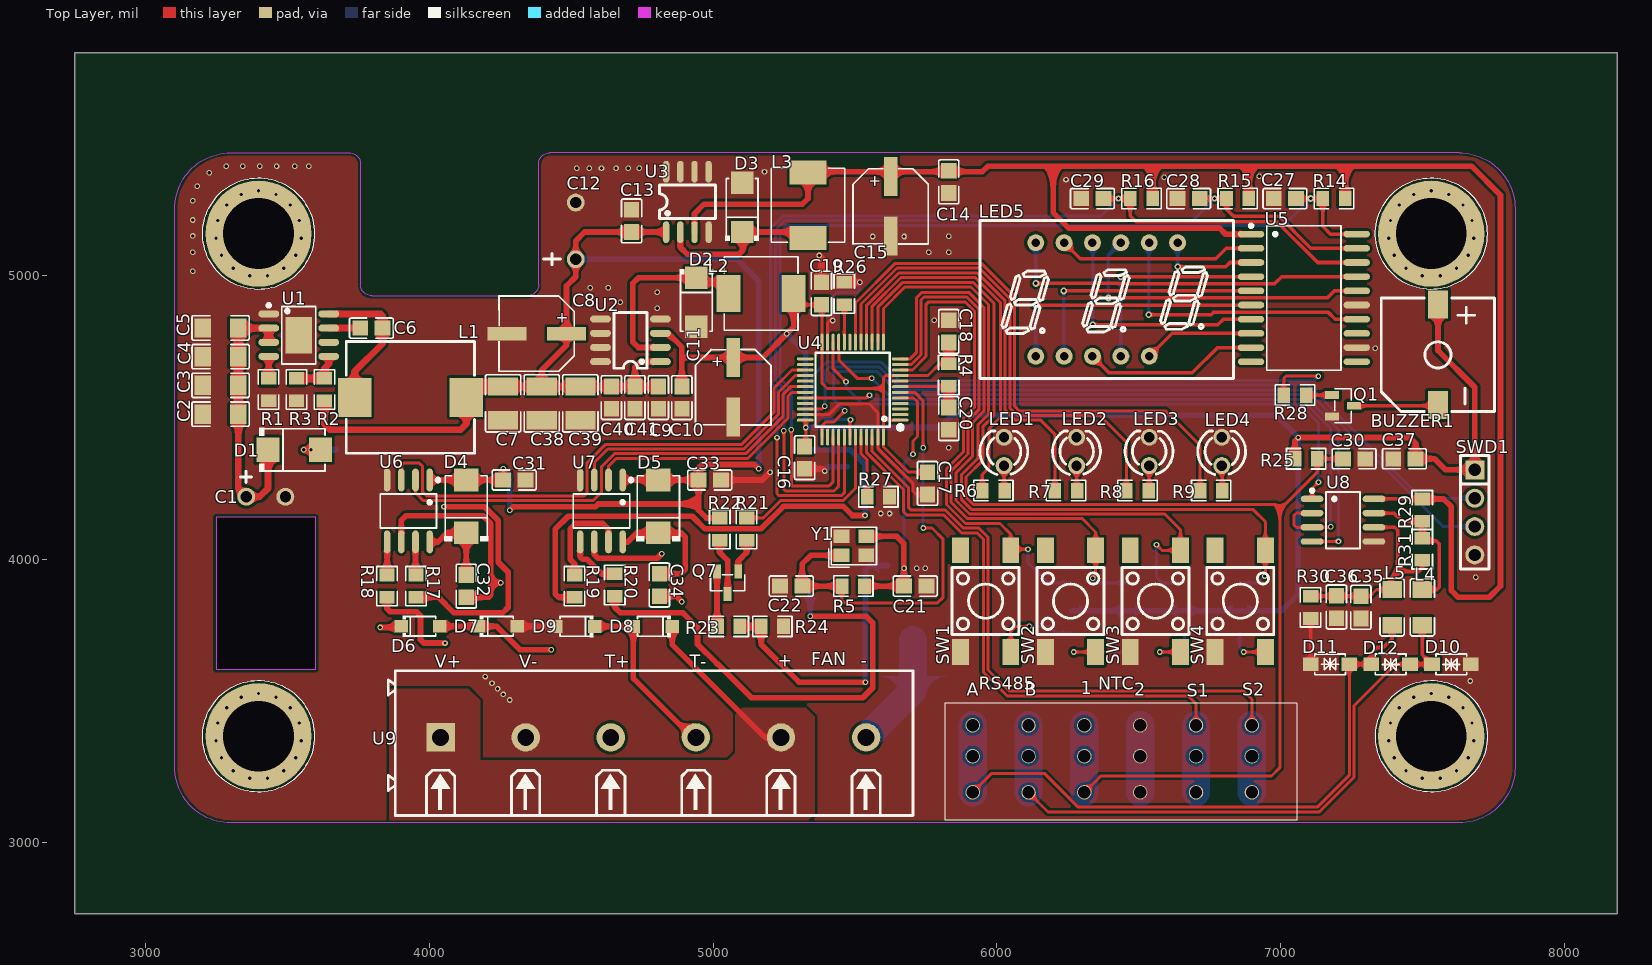
[diagram p0: Top Layer view]
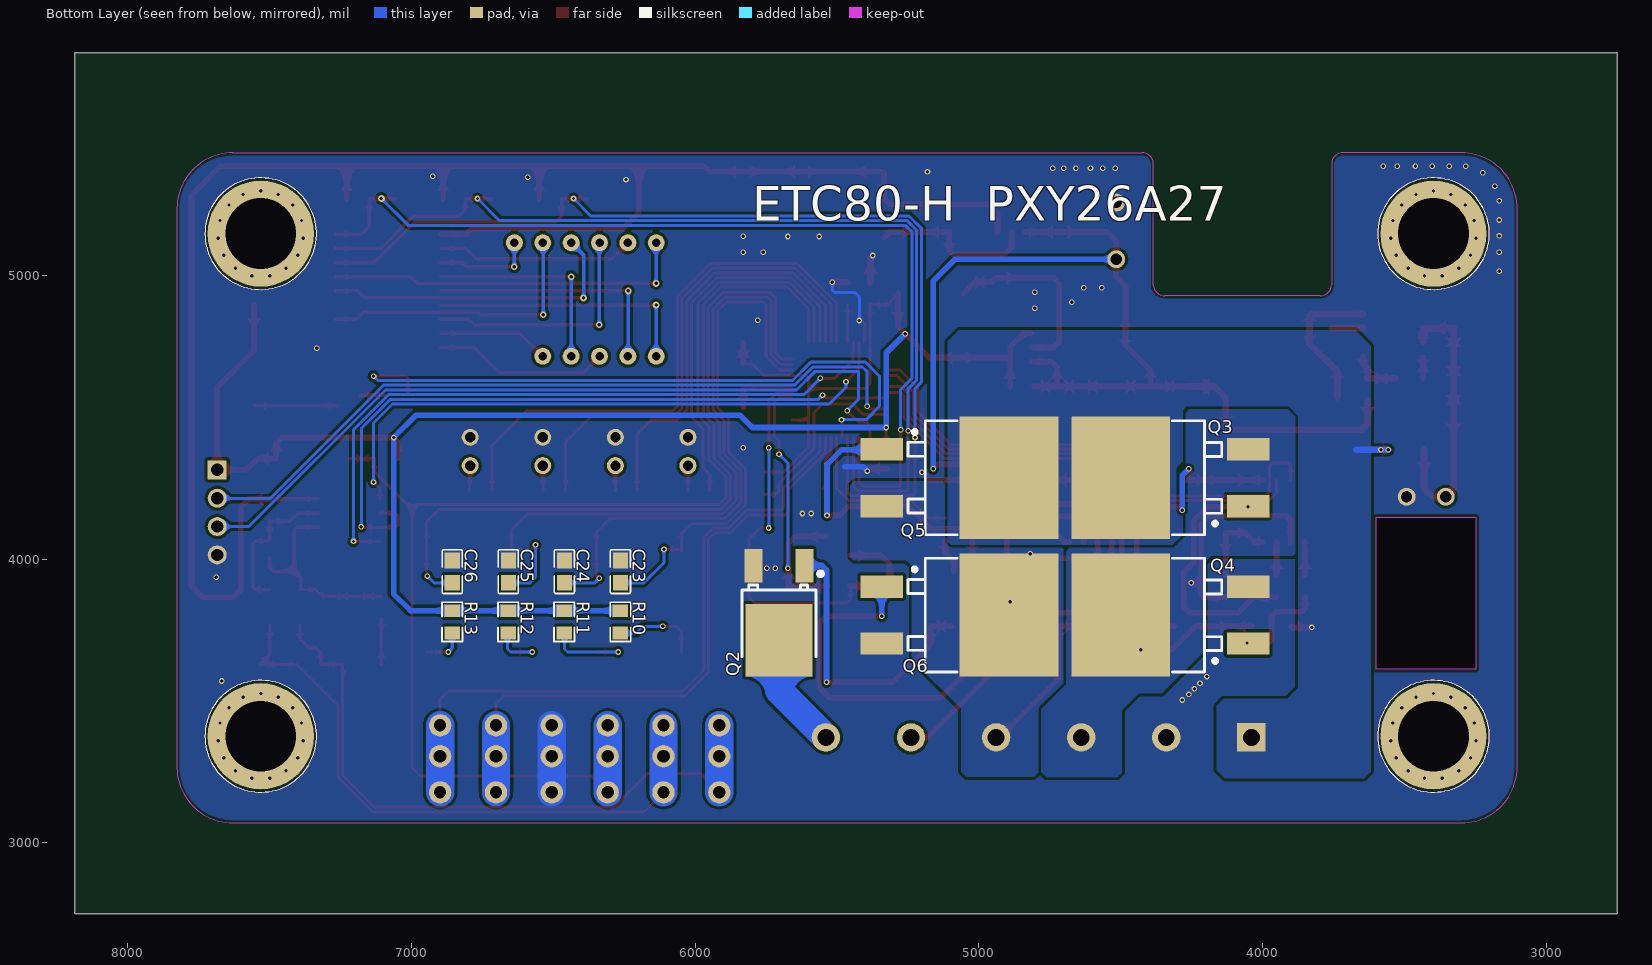
[diagram p1: Bottom Layer view, seen from below]
# Altium PCB MISC82093.pcbdoc (part 1 of 2)
Units mil, origin at the board's own origin, x right, y up, seen from the top; angles counter-clockwise.
Board outline 5437 x 3035.4 mil, 2 copper layers (Top Layer, Bottom Layer), stack 62.2 mil thick; 117 components, 84 nets, 389 pads, 166 vias.

## Layer stack, top to bottom
Top Solder Mask Layer: solder mask 0.4, Dk 3.3
Top Layer: signal copper 1.4
Dielectric1: surface 59.4, FR4, Dk 4.5
Bottom Layer: signal copper 1.4
Bottom Solder Mask Layer: solder mask 0.4, Dk 3.3

## Board outline
8187,2750 2750,2750 2750,5785.4 8187,5785.4
cut-out: 3248.1,4148.4 3248.1,3612.3 3598.7,3612.3 3598.7,4148.4

## Design rules (kind name [scope] priority, off if disabled: settings)
BoardOutlineClearance copperThickness1oz [All] p0: genericclearance=10 ignorepadtopadclearanceinfootprint=FALSE except(0: Arc-SplitContinuation Track-SplitContinuation SMDPad-SplitContinuation THPad-SplitContinuation Via-SplitContinuation Fill-SplitContinuation Poly-SplitContinuation Region-SplitContinuation Text-SplitContinuation)
BoardOutlineClearance copperThickness2oz [All] p0: genericclearance=10 ignorepadtopadclearanceinfootprint=FALSE except(0: Arc-SplitContinuation Track-SplitContinuation SMDPad-SplitContinuation THPad-SplitContinuation Via-SplitContinuation Fill-SplitContinuation Poly-SplitContinuation Region-SplitContinuation Text-SplitContinuation)
BoardOutlineClearance Plane_innerPlane [All] p0: genericclearance=10 ignorepadtopadclearanceinfootprint=FALSE except(0: Arc-SplitContinuation Track-SplitContinuation SMDPad-SplitContinuation THPad-SplitContinuation Via-SplitContinuation Fill-SplitContinuation Poly-SplitContinuation Region-SplitContinuation Text-SplitContinuation)
BoardOutlineClearance Copper_copperRegion [All] p0: genericclearance=10 ignorepadtopadclearanceinfootprint=FALSE except(0: Arc-SplitContinuation Track-SplitContinuation SMDPad-SplitContinuation THPad-SplitContinuation Via-SplitContinuation Fill-SplitContinuation Poly-SplitContinuation Region-SplitContinuation Text-SplitContinuation)
BoardOutlineClearance otherClearance [All] p0: genericclearance=10 ignorepadtopadclearanceinfootprint=FALSE except(0: Arc-SplitContinuation Track-SplitContinuation SMDPad-SplitContinuation THPad-SplitContinuation Via-SplitContinuation Fill-SplitContinuation Poly-SplitContinuation Region-SplitContinuation Text-SplitContinuation)
Clearance copperThickness1oz [All] p1: gap=7 ignorepadtopadclearanceinfootprint=FALSE
Clearance copperThickness2oz [All] p1: gap=7 ignorepadtopadclearanceinfootprint=FALSE
Clearance Plane_innerPlane [All] p1: gap=7 ignorepadtopadclearanceinfootprint=FALSE
Clearance Copper_copperRegion [All] p1: gap=7 ignorepadtopadclearanceinfootprint=FALSE
Clearance otherClearance [All] p1: gap=7 ignorepadtopadclearanceinfootprint=FALSE
DiffPairsRouting differentialPair [All] p1: maxuncoupledlength=10 minlimit=6 maxlimit=Infinity mostfreqgap=6 toplayer_minwidth=5 toplayer_prefwidth=10 toplayer_maxwidth=100 bottomlayer_minwidth=5 bottomlayer_prefwidth=10 bottomlayer_maxwidth=100
PasteMaskExpansion pasteMaskExpansion [All] p1: expansion=0
PlaneConnect innerPlane [All] p1: planeconnectstyle=Relief reliefexpansion=20 reliefentries=4 reliefconductorwidth=10 reliefairgap=10
PolygonConnect copperRegion [All] p1: connectstyle=Direct reliefentries=4 reliefconductorwidth=10 polygonreliefangle="90 Angle" airgapwidth=10
RoutingVias viaSize [All] p1: viastyle="Through Hole" holewidth=11.811 minholewidth=11.811 maxholewidth=248.0314 width=11.811 minwidth=11.811 maxwidth=248.0314
SolderMaskExpansion solderMaskExpansion [IsVia] p1: useseparateexpansions=TRUE expansion=-1000 expansionbottom=-1000
SolderMaskExpansion solderMaskExpansion [All] p2: useseparateexpansions=TRUE expansion=2 expansionbottom=2
Width copperThickness1oz [All] p1: maxlimit=120 minlimit=5 preferedwidth=10
Width copperThickness2oz [All] p1: maxlimit=100 minlimit=8 preferedwidth=10

## Components (designator, comment, footprint, x,y, rotation, side; value= is the part's Value field where it differs from the comment)
BUZZER1 "2.7kHz" BUZ-SMD_L9.6-W9.6-LS10.0-R 7555.1,4720.5 r90 top
C1 "33uF" CAP-TH_BD8.0-P3.50-D1.0-FD 3423.4,4220.5 r0 top
C2 "2.2uF" C1206 3263.8,4511.8 r0 top
C3 "2.2uF" C1206 3263.8,4613.1 r0 top
C4 "100nF" C1206 3263.8,4714.3 r0 top
C5 "100nF" C1206 3263.8,4815.6 r0 top
C6 "100nF" C0805#1 3795.3,4815 r0 top
C7 "22uF" C1210 4259.8,4549.7 r90 top
C8 "100uF" CAP-SMD_BD6.3-L6.6-W6.6-LS7.3-FD_JVS25V100M6X4#1 4378,4795.3 r180 top
C9 "100nF" C0805#1 4807.1,4570 r270 top
C10 "100nF" C0805#2 4889.8,4570 r90 top
C11 "100uF" CAP-SMD_BD6.3-L6.6-W6.6-LS7.3-FD_JVS25V100M6X4#2 5070.9,4606.3 r270 top
C12 "470uF" CAP-TH_BD10.0-P5.00-D1.0-FD 4515.7,5157.5 r0 top
C13 "100nF" C0805#3 4712.6,5192.9 r90 top
C14 "100nF" C0805#3 5830.7,5330.7 r90 top
C15 "100uF" CAP-SMD_BD6.3-L6.6-W6.6-LS7.3-FD_JVS25V100M6X4#2 5626,5244.1 r270 top
C16 "100nF" C0805#1 5322.8,4358.3 r90 top
C17 "100nF" C0805#3 5755.9,4267.7 r90 top
C18 "100nF" C0805#1 5830.7,4803.1 r270 top
C19 "100nF" C0805#3 5381.9,4937 r270 top
C20 "100nF" C0805#1 5830.7,4496.1 r90 top
C21 "22pF" C0805#3 5712.6,3905.5 r0 top
C22 "22pF" C0805#3 5275.6,3905.5 r180 top
C23 "100nF" C0805#3 6263.8,3956.6 r270 bottom
C24 "100nF" C0805#3 6461.4,3956.6 r270 bottom
C25 "100nF" C0805#3 6658.9,3956.6 r270 bottom
C26 "100nF" C0805#3 6856.5,3956.6 r270 bottom
C27 "100pF" C0805#1 7015.7,5271.7 r180 top
C28 "100pF" C0805#1 6676.4,5271.7 r180 top
C29 "100pF" C0805#3 6337.1,5271.7 r0 top
C30 "100nF" C0805#3 7259.8,4354.3 r0 top
C31 "10uF" C0805#3 4299.2,4279.5 r180 top
C32 "10uF" C0805#3 4129.9,3905.5 r90 top
C33 "10uF" C0805#3 4988.2,4279.5 r180 top
C34 "10uF" C0805#2 4811,3909.4 r90 top
C35 "100nF" C0805#3 7283.5,3830.7 r90 top
C36 "100nF" C0805#2 7197.5,3831.8 r270 top
C37 "100nF" C0805#3 7437,4354.3 r0 top
C38 "22uF" C1210 4395.9,4549.7 r90 top
C39 "22uF" C1210 4532,4549.7 r90 top
C40 "100nF" C0805#2 4641.5,4570 r90 top
C41 "1nF" C0805#2 4724.4,4570 r90 top
D1 "US2M-TP" SMB_L4.6-W3.6-LS5.3-RD#1 3523.6,4385.8 r0 top
D2 "SS34" SMA_L4.3-W2.6-LS5.2-RD#1 4940.9,4906 r270 top
D3 "SS34" SMA_L4.3-W2.6-LS5.2-RD#2 5102.4,5240.2 r90 top
D4 "MUR160SB" SMB_L4.6-W3.6-LS5.3-RD#2 4129.9,4186.6 r90 top
D5 "MUR160SB" SMB_L4.6-W3.6-LS5.3-RD#2 4807.1,4186.6 r90 top
D6 "RB160M-90" SOD-123FL_L2.7-W1.8-LS3.7-RD 3968.5,3763.8 r0 top
D7 "RB160M-90" SOD-123FL_L2.7-W1.8-LS3.7-RD 4241.5,3763.8 r0 top
D8 "RB160M-90" SOD-123FL_L2.7-W1.8-LS3.7-RD 4787.4,3763.5 r180 top
D9 "RB160M-90" SOD-123FL_L2.7-W1.8-LS3.7-RD 4514.4,3763.5 r180 top
D10 "SMF36CA" SOD-123_L2.7-W1.8-LS3.7-BI 7602.4,3629.9 r0 top
D11 "SMF36CA" SOD-123_L2.7-W1.8-LS3.7-BI 7174.6,3629.9 r180 top
D12 "SMF36CA" SOD-123_L2.7-W1.8-LS3.7-BI 7388.5,3629.9 r0 top
L1 "33uH" IND-SMD_L11.5-W10.0_FXL1040 3933.1,4570.9 r0 top
L2 "68uH" IND-SMD_L7.1-W6.6_H5.0#1 5169.3,4937 r180 top
L3 "68uH" IND-SMD_L7.1-W6.6_H5.0#2 5334.6,5248 r270 top
L4 "22uH" L1206 7500,3830.7 r270 top
L5 "22uH" L1206 7393.7,3830.7 r270 top
LED1 "3mmFIR" LED-TH_BD3.0-P2.54-FD 6025.6,4380.1 r90 top
LED2 "3mmFIR" LED-TH_BD3.0-P2.54-FD 6281.5,4380.1 r90 top
LED3 "3mmFIR" LED-TH_BD3.0-P2.54-FD 6537.4,4380.1 r90 top
LED4 "3mmFIR" LED-TH_BD3.0-P2.54-FD 6793.3,4380.1 r90 top
LED5 "SP420361N" LED-SEG-TH_SP420361N 6387.4,4915.9 r270 top
Q1 "SS8050(RANGE:200-350)" SOT-23-3_L2.9-W1.3-P1.90-LS2.4-BR 7220.5,4541.3 r180 top
Q2 "NCE0140K2-VB" TO-252-3_L6.6-W6.1-P4.58-LS10.1-BR 5704.7,3846.5 r90 bottom
Q3 "HYG025N06LS1B" TO-263-2_L10.2-W8.7-P5.08-LS15.1-BR 4275.6,4287.4 r180 bottom
Q4 "HYG025N06LS1B" TO-263-2_L10.2-W8.7-P5.08-LS15.1-BR 4275.6,3803.1 r180 bottom
Q5 "HYG025N06LS1B" TO-263-2_L10.2-W8.7-P5.08-LS15.1-BR 5118.1,4287.4 r0 bottom
Q6 "HYG025N06LS1B" TO-263-2_L10.2-W8.7-P5.08-LS15.1-BR 5118.1,3803.1 r0 bottom
Q7 "SS8050(RANGE:200-350)" SOT-23-3_L2.9-W1.3-P1.90-LS2.4-BR 5051.2,3917.3 r90 top
R1 "64.9kΩ" R0805#1 3433.1,4598.4 r90 top
R2 "100kΩ" R0805#2 3629.9,4598.4 r270 top
R3 "24.9kΩ" R0805#1 3531.5,4598.4 r90 top
R4 "10K" R0805#3 5830.7,4649.6 r90 top
R5 "1MΩ" R0805#3 5494.1,3905.5 r0 top
R6 "100Ω" R0805#3 5988.2,4242.1 r180 top
R7 "100Ω" R0805#3 6244.1,4242.1 r180 top
R8 "100Ω" R0805#1 6496.1,4242.1 r180 top
R9 "100Ω" R0805#3 6755.9,4242.1 r180 top
R10 "4.7kΩ" R0805#2 6263.8,3779.4 r270 bottom
R11 "4.7kΩ" R0805#2 6461.4,3779.4 r270 bottom
R12 "4.7kΩ" R0805#2 6658.9,3779.4 r270 bottom
R13 "4.7kΩ" R0805#2 6856.5,3779.4 r270 bottom
R14 "10K" R0805#3 7188.6,5271.7 r0 top
R15 "10K" R0805#3 6849.3,5271.7 r0 top
R16 "10K" R0805#2 6510,5271.7 r0 top
R17 "10Ω" R0805#3 3952.8,3905.5 r270 top
R18 "10Ω" R0805#3 3850.4,3905.5 r270 top
R19 "10Ω" R0805#3 4511.8,3905.5 r270 top
R20 "10Ω" R0805#2 4653.5,3909.4 r270 top
R21 "1kΩ" R0805#3 5118.1,4106.3 r270 top
R22 "4.7kΩ" R0805#3 5023.6,4106.3 r90 top
R23 "10Ω" R0805#3 5055.1,3763.6 r0 top
R24 "10K" R0805#2 5208.7,3763.6 r0 top
R25 "10K" R0805#1 7090.6,4354.3 r180 top
R26 "10K" R0805#3 5462.6,4937 r90 top
R27 "10K" R0805#2 5582.7,4220.5 r0 top
R28 "1kΩ" R0805#3 7051.2,4578.7 r0 top
R29 "47kΩ" R0805#1 7500,4173.2 r90 top
R30 "47kΩ" R0805#3 7106.3,3830.7 r90 top
R31 "120Ω" R0805#1 7500,4035.4 r90 top
SW1 "1TS005F-2600-9000A2-CT" SW-SMD_4P-L6.0-W6.0-P4.50-LS9.0-2#1 5960.6,3852.5 r90 top
SW2 "1TS005F-2600-9000A2-CT" SW-SMD_4P-L6.0-W6.0-P4.50-LS9.0-2#1 6259.8,3852.5 r90 top
SW3 "1TS005F-2600-9000A2-CT" SW-SMD_4P-L6.0-W6.0-P4.50-LS9.0-2#2 6559.1,3852.5 r90 top
SW4 "1TS005F-2600-9000A2-CT" SW-SMD_4P-L6.0-W6.0-P4.50-LS9.0-2#3 6858.3,3852.5 r90 top
SWD1 "220S-1*4P H=8.5MM Ytype Gold-plated" DIP-1X4P2.54 7685,4165.4 r270 top
U1 "LMR38020SDDAR" ESOP-8_L4.9-W3.9-P1.27-LS6.0-BL-EP-1 3539.4,4790 r270 top
U2 "XL1509-3.3E1" SOP-8_L4.9-W3.9-P1.27-LS6.0-BL 4708.7,4771.7 r90 top
U3 "XL1509-5.0E1" SOIC-8_L5.0-W4.0-P1.27-LS6.0-BL 4909.4,5259.8 r0 top
U4 "STM32F103C8T6" LQFP-48_L7.0-W7.0-P0.50-LS9.0-BL 5492.1,4598.4 r90 top
U5 "TM1620" SOIC-20_L13.0-W7.6-P1.27-LS10.3-BL 7082.7,4921.3 r270 top
U6 "IR2103STRPBF" SOIC-8_L4.9-W3.9-P1.27-LS6.0-BL 3925.9,4170.4 r180 top
U7 "IR2103STRPBF" SOIC-8_L4.9-W3.9-P1.27-LS6.0-BL 4606.3,4170.4 r180 top
U8 "MAX485ESA(UMW)" SOP-8_L5.0-W4.0-P1.27-LS6.0-BL 7220.5,4137.8 r270 top
U9 "KF7620-7.62-6P" CONN-TH_6P-P7.62_KF7620-7.62-6P 4789.4,3372.2 r0 top
Y1 "8MHz" CRYSTAL-SMD_4P-L3.2-W2.5-BL 5496.1,4047.2 r0 top

## Footprints (in the part's own frame and the unit in brackets; to place one, negate y for a bottom-side part, rotate by r counter-clockwise, add the part's x,y. Pads: shape width x height; smd on the part's side, far side on the other; paste and mask are expansions set on the pad)
BUZ-SMD_L9.6-W9.6-LS10.0-R [mil]
  rect 98.4x70.9 smd: 1(177.2,0) 2(-177.2,0)
  silkscreen extent -200,-200 200,200
C0805#1 [mil]
  rect 55.5x53.1 smd paste-3937 mask+2: 1(-39.4,0) 2(39.3,0)
  silkscreen extent -77,-36 77,36
C0805#2 [mil]
  rect 55.5x53.1 smd paste-3937 mask+2: 1(-39.3,0) 2(39.4,0)
  silkscreen extent -77,-36 77,36
C0805#3 [mil]
  rect 55.5x53.1 smd paste-3937 mask+2: 1(-39.4,0) 2(39.4,0)
  silkscreen extent -77,-36 77,36
C1206 [mil]
  rect 58.5x68 smd paste-3937 mask+2: 1(-62.7,0) 2(62.7,0)
  silkscreen extent -101,-43 101,43
C1210 [mil]
  rect 64.4x106.3 smd paste-3937 mask+2: 1(-59.8,0) 2(59.7,0)
  silkscreen extent -101,-62 101,62
CAP-SMD_BD6.3-L6.6-W6.6-LS7.3-FD_JVS25V100M6X4#1 [mil]
  rect 137.8x47.2 smd: 1(-105.1,0) 2(105.2,0)
  silkscreen extent -133,-133 133,133
CAP-SMD_BD6.3-L6.6-W6.6-LS7.3-FD_JVS25V100M6X4#2 [mil]
  rect 137.8x47.2 smd: 1(-105.1,0) 2(105.1,0)
  silkscreen extent -133,-133 133,133
CAP-TH_BD8.0-P3.50-D1.0-FD [mil]
  round 63 hole 39.4: 1(-68.9,0) 2(68.9,0)
  silkscreen extent -90,50 -50,90
CAP-TH_BD10.0-P5.00-D1.0-FD [mil]
  round 63 hole 39.4: 1(0,-100) 2(0,100)
  silkscreen extent -114,-119 -54,-79
CONN-TH_6P-P7.62_KF7620-7.62-6P [mil]
  rect 100x100 hole 59.1: 1(-750,0)
  round 100 hole 59.1: 2(-450,0) 3(-150,0) 4(150,0) 5(450,0) 6(750,0)
  silkscreen extent -934,-275 915,235
CRYSTAL-SMD_4P-L3.2-W2.5-BL [mil]
  rect 55.1x47.2 smd: 1(-43.3,-33.4) 2(43.3,-33.4) 3(43.3,33.5) 4(-43.3,33.5)
  silkscreen extent -89,-75 80,66
DIP-1X4P2.54 [mil]
  rect 66.9x66.9 hole 43.3: 1(-150,0)
  round 66.9 hole 43.3: 2(-50,0) 3(50,0) 4(150,0)
  silkscreen extent -200,-50 200,50
ESOP-8_L4.9-W3.9-P1.27-LS6.0-BL-EP-1 [mil]
  oval 24.8x73.4 smd: 1(-75,-105.6) 2(-25,-105.6) 3(25,-105.6) 4(75,-105.6) 5(75,105.6) 6(25,105.6) 7(-25,105.6) 8(-75,105.6)
  rect 129.9x94.5 smd paste+0 mask+2: 9(0,0)
  silkscreen extent -111,-112 102,60
IND-SMD_L7.1-W6.6_H5.0#1 [mil]
  rect 84.6x130.7 smd: 1(-114.7,0) 2(114.7,0)
  silkscreen extent -130,-130 130,130
IND-SMD_L7.1-W6.6_H5.0#2 [mil]
  rect 84.6x130.7 smd: 1(-114.7,0) 2(114.6,0)
  silkscreen extent -130,-130 130,130
IND-SMD_L11.5-W10.0_FXL1040 [mil]
  rect 118.1x137.8 smd: 1(-196.9,0) 2(196.8,0)
  silkscreen extent -226,-197 226,197
L1206 [mil]
  rect 58.5x68 smd paste-3937 mask+2: 1(-62.7,0) 2(62.7,0)
  silkscreen extent -101,-43 101,43
LED-SEG-TH_SP420361N [mil]
  round 60 hole 30: 1(200,-250) 2(200,-150) 3(200,-50) 4(200,50) 5(200,150) 7(-200,250) 8(-200,150) 9(-200,50) 10(-200,-50) 11(-200,-150) 12(-200,-250)
  silkscreen extent -279,-447 279,447
LED-TH_BD3.0-P2.54-FD [mil]
  round 60 hole 36: 1(-50,0) 2(50,0)
  silkscreen extent -81,-84 72,85
LQFP-48_L7.0-W7.0-P0.50-LS9.0-BL [mil]
  oval 10.6x59.1 smd paste+0 mask+2: 1(-108.2,-167.3) 2(-88.6,-167.3) 3(-68.9,-167.3) 4(-49.2,-167.3) 5(-29.5,-167.3) 6(-9.8,-167.3) 7(9.9,-167.3) 8(29.6,-167.3) 9(49.2,-167.3) 10(68.9,-167.3) 11(88.6,-167.3) 12(108.3,-167.3) 25(108.3,167.3) 26(88.6,167.3) 27(68.9,167.3) 28(49.2,167.3) 29(29.6,167.3) 30(9.9,167.3) 31(-9.8,167.3) 32(-29.5,167.3) 33(-49.2,167.3) 34(-68.9,167.3) 35(-88.6,167.3) 36(-108.2,167.3)
  oval 59.1x10.6 smd paste+0 mask+2: 13(167.3,-108.3) 14(167.3,-88.6) 15(167.3,-68.9) 16(167.3,-49.2) 17(167.3,-29.6) 18(167.3,-9.9) 19(167.3,9.8) 20(167.3,29.5) 21(167.3,49.2) 22(167.3,68.9) 23(167.3,88.6) 24(167.3,108.2) 37(-167.3,108.2) 38(-167.3,88.6) 39(-167.3,68.9) 40(-167.3,49.2) 41(-167.3,29.5) 42(-167.3,9.8) 43(-167.3,-9.9) 44(-167.3,-29.6) 45(-167.3,-49.2) 46(-167.3,-68.9) 47(-167.3,-88.6) 48(-167.3,-108.3)
  silkscreen extent -141,-176 130,132
R0805#1 [mil]
  rect 44.6x54.2 smd paste-3937 mask+2: 1(-39.3,0) 2(39.4,0)
  silkscreen extent -69,-36 69,36
R0805#2 [mil]
  rect 44.6x54.2 smd paste-3937 mask+2: 1(-39.4,0) 2(39.3,0)
  silkscreen extent -69,-36 69,36
R0805#3 [mil]
  rect 44.6x54.2 smd paste-3937 mask+2: 1(-39.4,0) 2(39.4,0)
  silkscreen extent -69,-36 69,36
SMA_L4.3-W2.6-LS5.2-RD#1 [mil]
  rect 78.7x78.7 smd: 1(-86.6,0) 2(86.6,0)
  silkscreen extent -117,-59 102,59
SMA_L4.3-W2.6-LS5.2-RD#2 [mil]
  rect 78.7x78.7 smd: 1(-86.7,0) 2(86.6,0)
  silkscreen extent -117,-59 102,59
SMB_L4.6-W3.6-LS5.3-RD#1 [mil]
  rect 80.6x86.3 smd: 1(-92.9,0) 2(93,0)
  silkscreen extent -123,-77 108,77
SMB_L4.6-W3.6-LS5.3-RD#2 [mil]
  rect 80.6x86.3 smd: 1(-93,0) 2(92.9,0)
  silkscreen extent -123,-77 108,77
SOD-123_L2.7-W1.8-LS3.7-BI [mil]
  rect 55.1x47.2 smd: 1(-68.3,0) 2(68.3,0)
  silkscreen extent -54,-36 54,36
SOD-123FL_L2.7-W1.8-LS3.7-RD [mil]
  rect 47.2x45.3 smd: 1(-68.3,0) 2(68.3,0)
  silkscreen extent -63,-38 54,38
SOIC-8_L4.9-W3.9-P1.27-LS6.0-BL [mil]
  oval 23.1x80.5 smd: 1(-75,-109.1) 2(-25,-109.1) 3(25,-109.1) 4(75,-109.1) 5(75,109.2) 6(25,109.2) 7(-25,109.2) 8(-75,109.2)
  silkscreen extent -110,-115 100,60
SOIC-8_L5.0-W4.0-P1.27-LS6.0-BL [mil]
  oval 22.4x76.8 smd: 1(-75,-106.5) 2(-25,-106.5) 3(25,-106.5) 4(75,-106.5) 5(75,106.5) 6(25,106.5) 7(-25,106.5) 8(-75,106.5)
  silkscreen extent -98,-59 98,59
SOIC-20_L13.0-W7.6-P1.27-LS10.3-BL [mil]
  oval 23.4x92.9 smd: 1(-225,-186.2) 2(-175,-186.2) 3(-125,-186.2) 4(-75,-186.2) 5(-25,-186.2) 6(25,-186.2) 7(75,-186.2) 8(125,-186.2) 9(175,-186.2) 10(225,-186.2) 11(225,186.2) 12(175,186.2) 13(125,186.2) 14(75,186.2) 15(25,186.2) 16(-25,186.2) 17(-75,186.2) 18(-125,186.2) 19(-175,186.2) 20(-225,186.2)
  silkscreen extent -260,-192 255,131
SOP-8_L4.9-W3.9-P1.27-LS6.0-BL [mil]
  oval 24.8x73.4 smd: 1(-75,-105.6) 2(-25,-105.6) 3(25,-105.6) 4(75,-105.6) 5(75,105.6) 6(25,105.6) 7(-25,105.6) 8(-75,105.6)
  silkscreen extent -98,-59 98,58
SOP-8_L5.0-W4.0-P1.27-LS6.0-BL [mil]
  oval 22.6x80.1 smd: 1(-75,-109) 2(-25,-109) 3(25,-109) 4(75,-109) 5(75,108.9) 6(25,108.9) 7(-25,108.9) 8(-75,108.9)
  silkscreen extent -110,-115 100,60
SOT-23-3_L2.9-W1.3-P1.90-LS2.4-BR [mil]
  rect 49.2x27.6 smd: 1(39.4,-37.4) 2(39.4,37.4) 3(-39.3,0)
  silkscreen extent -29,-60 29,60
SW-SMD_4P-L6.0-W6.0-P4.50-LS9.0-2#1 [mil]
  rect 90.6x59.1 smd: 1(-179.1,88.5) 2(179.1,88.5) 3(-179.1,-88.6) 4(179.1,-88.6)
  silkscreen extent -118,-118 118,118
SW-SMD_4P-L6.0-W6.0-P4.50-LS9.0-2#2 [mil]
  rect 90.6x59.1 smd: 1(-179.1,88.6) 2(179.1,88.6) 3(-179.1,-88.5) 4(179.1,-88.5)
  silkscreen extent -118,-118 118,118
SW-SMD_4P-L6.0-W6.0-P4.50-LS9.0-2#3 [mil]
  rect 90.6x59.1 smd: 1(-179.1,88.6) 2(179.1,88.6) 3(-179.1,-88.6) 4(179.1,-88.6)
  silkscreen extent -118,-118 118,118
TO-252-3_L6.6-W6.1-P4.58-LS10.1-BR [mil]
  rect 118.1x63 smd: 1(131.6,-89.9) 2(131.6,90)
  rect 255.9x236.2 smd: 3(-131.6,0)
  silkscreen extent -190,-154 110,130
TO-263-2_L10.2-W8.7-P5.08-LS15.1-BR [mil]
  rect 150x78.7 smd: 1(224.6,-100) 3(224.6,100)
  rect 348x433.1 smd: 4(-224.5,0)
  silkscreen extent -41,-201 132,201

## Free pads (board coordinates)
  round 51.2 / inner round 51.2 / far side round 78.7 hole 43.3 paste+0 mask+4: 0(5915,3178.4) 0(5915,3414.6) 0(6111.9,3178.4) 0(6111.9,3414.6) 0(6308.7,3178.4) 0(6308.7,3414.6) 0(6505.6,3178.4) 0(6505.6,3414.6) 0(6702.4,3178.4) 0(6702.4,3414.6) 0(6899.3,3178.4) 0(6899.3,3414.6)
  round 374 hole 250: 1(3397.6,3376.1) 1(3397.6,5147.8) 1(7531.5,3376.1) 1(7531.5,5147.8)
  round 51.2 / inner round 51.2 / far side round 78.7 hole 45 paste+0 mask+4: 1(5915,3305.9) 2(6111.9,3305.9) 3(6308.7,3305.9) 3(6702.4,3305.9) 4(6505.6,3305.9) 4(6899.3,3305.9)

## Via types
v1: diameter 19.7, hole 11.8, Top Layer to Bottom Layer, 157 vias
v2: diameter 24, hole 12, Top Layer to Bottom Layer, 9 vias

## Nets (pads, with @x,y where several pads share a name; then routed paths per layer and width w, separated by ;. In a path a pad name is that pad's centre, name@x,y a point inside that pad or via, vN(x,y) a via of type N, cw(c..) or ccw(c..) an arc to the next point about the centre after c; other vN are vias at no path point)
1: LED5.12 U5.17 | length 1285.3
  Top Layer w12.5: v2(6137.8,4972.4) 6426.5,4972.4 6427,4972 6979.9,4972 7004.1,4996.3 U5.17@7268.9,4996.3
  Bottom Layer w12.5: LED5.12@6137.4,5116.2 6137.8,5115.8 v2(6137.8,4972.4)
2: LED5.9 U5.16 | length 1098.6
  Top Layer w12.5: v2(6393.7,4921.3) 7165.4,4921.3 7190.4,4946.3 U5.16@7268.9,4946.3
  Bottom Layer w12.5: v2(6393.7,4921.3) 6393.7,5072.6 LED5.9@6437.4,5116.2
3: LED5.8 U5.14 | length 1001.6
  Top Layer w12.5: v2(6535.4,4862.2) 6755.9,4862.2 6763.9,4870.2 7169.2,4870.2 7193.1,4846.3 U5.14@7268.9,4846.3
  Bottom Layer w12.5: v2(6535.4,4862.2) 6535.4,5114.3 LED5.8@6537.4,5116.2
$1N16317: C6.2 L1.1 U1.8 | length 520.6
  Top Layer w23.6: U1.8@3645,4865 3828,4865 3834.6,4858.3 C6.2@3834.6,4815 3834.6,4759.8 3736.2,4661.4 L1.1@3736.2,4570.9
$1N16318: C6.1 U1.7 | length 110.9
  Top Layer w23.6: U1.7@3645,4815 C6.1@3755.9,4815
$1N16321: R1.2 U1.4 | length 74.9
  Top Layer w20: R1.2@3433.1,4637.8 3433.8,4638.5 U1.4@3433.8,4712.4
$1N16326: R2.1 R3.2 U1.5 | length 181.9
  Top Layer w23.6: R3.2@3531.5,4637.8 R2.1@3629.9,4637.8 3629.9,4673.2 3645,4688.3 U1.5@3645,4715
$1N16330: C32.2 D4.1 U6.8 | length 291.1
  Top Layer w20: U6.8@4000.9,4061.2 4029.7,4061.2 4062.2,4093.6 D4.1@4129.9,4093.6 C32.2@4129.9,3944.9
$1N16331: R17.1 U6.7 | length 117.1
  Top Layer w20: U6.7@3950.9,4061.2 3950.9,3946.8 R17.1@3952.8,3944.9
$1N16333: R18.1 U6.5 | length 116.5
  Top Layer w20: R18.1@3850.4,3944.9 3850.9,3945.4 U6.5@3850.9,4061.2
$1N16334: Q4.1 R18.2 | length 344.2
  Top Layer w20: R18.2@3850.4,3866.1 3850.4,3826.8 3862.2,3815 3954.7,3815 3968.5,3801.2 3968.5,3716.5 3980.3,3704.7 v1(4055.1,3704.7)
$1N16337: C34.2 D5.1 U7.8 | length 451.1
  Top Layer w20: U7.8@4681.3,4061.2 4699,4061.2 4731.4,4093.6 D5.1@4807.1,4093.6 4886.7,4093.6 4901.6,4078.7 4901.6,3964.6 4885.8,3948.8 C34.2@4811,3948.8
$1N16338: R19.1 U7.7 | length 364.4
  Top Layer w20: R19.1@4511.8,3944.9 4511.8,3984.3 4496.1,4000 4496.1,4106.3 4515.7,4126 4611.3,4126 4631.3,4106 U7.7@4631.3,4061.2
$1N16340: R20.1 U7.5 | length 199.9
  Top Layer w20: U7.5@4531.3,4061.2 4531.3,4008.1 4539.4,4000 4555.1,4000 4606.3,3948.8 R20.1@4653.5,3948.8
$1N16341: Q5.1 R19.2 | length 1871.8
  Top Layer w20: R19.2@4511.8,3866.1 4455.1,3866.1 4443.3,3878 4443.3,4106.1 4489.2,4152 4926.8,4152 4971.3,4107.4 5169,4107.4 5248.1,4186.5 5459.2,4186.5 5491,4154.6 v1(5535.4,4154.6)
  Bottom Layer w20: Q5.1@5342.7,4387.4 5344.2,4385.8 5484.3,4385.8 5535.4,4334.6 v1(5535.4,4154.6)
$1N16342: Q6.1 R20.2 | length 1692.9
  Top Layer w20: R20.2@4653.5,3870.1 4653.5,3830.7 4673.2,3811 4893.7,3811 4944.9,3759.8 4944.9,3700.8 5013.4,3632.3 5014.7,3632.3 5135.2,3511.8 5527.6,3511.8 5563,3547.2 5563,3775.6 5539.4,3799.2 v1(5342.5,3799.2)
  Bottom Layer w20: v1(5342.5,3799.2) 5342.5,3903 Q6.1@5342.7,3903.1
$1N16417: BUZZER1.2 Q1.3 | length 296.2
  Top Layer w12.5: Q1.3@7259.8,4541.3 7553.2,4541.3 BUZZER1.2@7555.1,4543.3
$1N16473: C20.2 R4.1 U4.7 | length 246.9
  Top Layer w10.6: U4.7@5659.4,4608.3 5828.7,4608.3 R4.1@5830.7,4610.2
  Top Layer w20: C20.2@5830.7,4535.4 R4.1@5830.7,4610.2
$1N16482: R10.2 SW1.3 | length 304.4
  Top Layer w10.6: SW1.3@6049.2,3673.4 6049.2,3746.1 6066.9,3763.8 v1(6114.2,3763.8)
  Bottom Layer w10.6: v1(6114.2,3763.8) 6185,3763.8 6208.8,3740.1 R10.2@6263.8,3740.1
$1N16483: R11.2 SW2.3 | length 312
  Top Layer w10.6: v1(6271.7,3673.2) 6348.3,3673.2 SW2.3@6348.4,3673.4
  Bottom Layer w10.6: v1(6271.7,3673.2) 6450,3673.2 6460.6,3683.9 R11.2@6460.6,3725.7
$1N16484: R12.2 SW3.3 | length 219.2
  Top Layer w10.6: v1(6574.8,3673.2) 6647.5,3673.2 SW3.3@6647.6,3673.4
  Bottom Layer w10.6: v1(6574.8,3673.2) 6650.8,3673.2 6661.4,3683.9 R12.2@6661.4,3739.1
$1N16495: R13.2 SW4.3 | length 149.4
  Top Layer w10.6: v1(6870.1,3673.2) 6946.7,3673.2 SW4.3@6946.9,3673.4
  Bottom Layer w10.6: R13.2@6856.5,3740.1 6856.5,3686.8 v1(6870.1,3673.2)
$1N16508: Q3.1 R17.2 | length 888.1
  Top Layer w20: R17.2@3952.8,3866.1 4031.5,3866.1 4086.6,3811 4258,3811 4278,3831 4278,3954.3 4242.5,3989.7 4242.5,4136.8 4194.2,4185 v1(4051.2,4185)
$1N21222: D2.1 L2.2 U2.2 | length 681.4
  Top Layer w20: U2.2@4814.3,4746.7 4736.5,4746.7 4716.5,4766.7 4716.5,4972.6 4736.5,4992.6 D2.1@4940.9,4992.6 4956.7,4976.9 5014.7,4976.9 L2.2@5054.6,4937
$1N21228: D3.1 L3.2 U3.2 | length 596
  Top Layer w20: U3.2@4884.4,5153.3 4884.4,5099.8 4909.4,5074.8 5090.6,5074.8 5104.7,5088.9 5104.7,5151.2 D3.1@5102.4,5153.5 5314.4,5153.5 L3.2@5334.6,5133.4
$1N21236: LED1.1 R6.1 | length 88.8
  Top Layer w10.6: LED1.1@6025.6,4330.1 6025.6,4244.1 R6.1@6027.6,4242.1
$1N21238: LED2.1 R7.1 | length 88.8
  Top Layer w10.6: LED2.1@6281.5,4330.1 6281.5,4244.1 R7.1@6283.5,4242.1
$1N21240: LED3.1 R8.1 | length 88.8
  Top Layer w10.6: R8.1@6535.4,4242.1 6537.4,4244.1 LED3.1@6537.4,4330.1
$1N21242: LED4.1 R9.1 | length 88.8
  Top Layer w10.6: LED4.1@6793.3,4330.1 6795.3,4328.1 R9.1@6795.3,4242.1
$1N21243: Q1.1 R28.2 | length 90.5
  Top Layer w12.5: R28.2@7090.6,4578.7 Q1.1@7181.1,4578.7
$1N21245: Q7.2 R23.1 | length 193.9
  Top Layer w20: Q7.2@5013.8,3956.7 5013.8,3765.6 R23.1@5015.7,3763.6
$1N21249: Q7.1 R21.2 | length 122.4
  Top Layer w20: Q7.1@5088.6,3956.7 5088.6,3994.1 5118.1,4023.6 R21.2@5118.1,4066.9
$1N21273: C35.2 C36.1 L5.1 R30.2 R31.1 U8.6 | length 734.1
  Top Layer w10.6: C35.2@7283.5,3870.1 7315,3870.1 7338.3,3893.4 L5.1@7393.7,3893.4
  Top Layer w12.5: R30.2@7106.3,3870.1 C35.2@7283.5,3870.1 ; U8.6@7329.4,4112.8 7403,4112.8 7413.4,4102.4 7413.4,3956.7 ; L5.1@7393.7,3893.4 7389.8,3897.3 7389.8,3933.1 7413.4,3956.7 ; R31.1@7500,4005.8 7500,3969.2 7487.5,3956.7 7413.4,3956.7
$1N21274: L4.1 R29.1 R31.2 U8.7 | length 530.6
  Top Layer w12.5: U8.7@7329.4,4162.8 7400.2,4162.8 7429.1,4133.9 R29.1@7500,4133.9 7500,4065.1 7549.1,4065.1 7559.1,4055.1 7559.1,3901.6 7550.9,3893.4 L4.1@7500,3893.4
$1N21282: Q2.1 R23.2 R24.1 | length 1040.5
  Top Layer w20: R23.2@5094.5,3763.6 R24.1@5169.3,3763.6 5169.3,3700.8 5303.1,3566.9 v1(5537,3566.9)
  Bottom Layer w20: v1(5537,3566.9) 5537,3962.2 5552.9,3978.1 Q2.1@5614.8,3978.1
$1N21294: Q7.3 R22.1 | length 200.4
  Top Layer w20: R22.1@5023.6,4066.9 5023.6,4023.6 5051.2,3996.1 Q7.3@5051.2,3878
$1N21299: C1.1 C2.2 C3.2 C4.2 C5.2 D1.1 U1.2 U1.3 | length 988.7
  Top Layer w23.6: D1.1@3430.7,4385.8 3430.7,4249.6 3401.6,4220.5 C1.1@3354.5,4220.5 3326.5,4248.5 C2.2@3326.5,4511.8 C3.2@3326.5,4613.1 C4.2@3326.5,4714.3 C5.2@3326.5,4815.6 3327.1,4815 U1.2@3433.8,4815 U1.3@3433.8,4765
+3.3V: BUZZER1.1 C10.2 C11.1 C16.2 C17.2 C18.2 C19.2 C37.2 L2.1 R4.2 R10.1 R11.1 R12.1 R13.1 R25.2 SWD1.1 U2.3 U4.1 U4.9 U4.24 U4.36 U4.48 | length 7267.5
  Top Layer w10.6: L2.1@5284,4937 5323.3,4897.6 5383.9,4897.6 U4.24@5383.9,4765.7 5383.9,4620.1 5401.6,4602.4 5600.4,4602.4 ; C16.2@5322.8,4397.6 5326.8,4401.6 v1(5326.8,4464.6) 5326.8,4488.2 U4.36@5324.8,4490.2 ; U4.1@5659.4,4490.2 5604.3,4490.2 5600.4,4486.2 ; C17.2@5755.9,4307.1 5689,4307.1 5600.4,4395.7 U4.48@5600.4,4431.1 5600.4,4486.2 ; R4.2@5830.7,4689 5799.2,4689 5757.9,4647.6 U4.9@5659.4,4647.6 5608.3,4647.6 5600.4,4639.8 5600.4,4602.4 ; 5600.4,4486.2 5600.4,4602.4
  Top Layer w20: U2.3@4814.3,4796.7 4841.1,4796.7 4889.8,4748 4889.8,4700.8 ; C10.2@4889.8,4609.4 4889.8,4700.8 ; L2.1@5284,4937 5284,4819.4 v1(5259.8,4795.3) 5176,4711.4 C11.1@5070.9,4711.4 4900.4,4711.4 4889.8,4700.8 ; R4.2@5830.7,4689 C18.2@5830.7,4763.8 ; R25.2@7051.2,4354.3 7051.2,4417.3 v1(7063,4429.1) 7456.7,4429.1 7476.4,4409.4 C37.2@7476.4,4354.3 7543.3,4354.3 7582.3,4315.4 SWD1.1@7685,4315.4 7685,4606.3 7555.1,4736.2 BUZZER1.1@7555.1,4897.7
  Bottom Layer w20: v1(5259.8,4795.3) 5326.8,4728.3 v1(5326.8,4464.6) 5799.2,4464.6 5842.5,4507.9 6984.3,4507.9 v1(7063,4429.1) 7063,3878 7003.9,3818.9 R13.1@6856.5,3818.9 ; R10.1@6263.8,3818.8 R11.1@6461.4,3818.8 6658.9,3818.9 6856.4,3818.9 R13.1@6856.5,3818.8
+5V: C14.2 C15.1 L3.1 R14.2 R15.2 R16.2 R29.2 U3.3 U5.1 U8.8 | length 6464.1
  Top Layer w12.5: U8.8@7329.4,4212.8 7499.8,4212.8 R29.2@7500,4212.6
  Top Layer w20: U3.3@4934.4,5153.3 4934.4,5217.9 4968.5,5252 5314.6,5252 5334.6,5272 L3.1@5334.6,5362.7 5338.4,5366.5 5949.1,5366.5 5968.5,5385.8 6198.5,5385.8 ; R16.2@6549.3,5271.7 6549.3,5385.1 6550,5385.8 ; R15.2@6888.7,5271.7 6888.7,5385.4 6889.1,5385.8 ; U5.1@6896.5,5146.3 6895.9,5145.7 6807.1,5145.7 6784.9,5167.9 6253.4,5167.9 6198.5,5222.8 6198.5,5385.8 ; R14.2@7228,5271.7 7228,5385.1 7228.7,5385.8 ; R29.2@7500,4212.6 7574.8,4212.6 7602.4,4185 7602.4,3889.8 7626,3866.1 7736.2,3866.1 7775.6,3905.5 7775.6,5283.5 7673.2,5385.8 7228.7,5385.8 ; 6198.5,5385.8 6550,5385.8 ; 6550,5385.8 6889.1,5385.8 ; 6889.1,5385.8 7228.7,5385.8
+12V: C7.2 C8.1 C9.1 C12.1 C13.1 C31.2 C33.2 C38.2 C39.2 C40.2 C41.2 D4.2 D5.2 L1.2 R2.2 R22.2 U2.1 U3.1 U6.1 U7.1 | length 5652.6
  Top Layer w20: U6.1@4000.9,4279.5 D4.2@4129.9,4279.5 C31.2@4259.8,4279.5 ; v1(4259.8,4318.9) C31.2@4259.8,4279.5 ; C7.2@4259.8,4609.4 C38.2@4392,4609.4 ; C31.2@4279.5,4279.5 C31.2@4259.8,4279.5 ; v1(4283.5,4173.2) 4295.3,4185 4585.3,4185 4594.9,4194.7 4948.8,4194.7 ; C39.2@4528.1,4609.4 C38.2@4395.9,4609.4 4395.9,4667.6 4483.1,4754.7 C8.1@4483.1,4795.3 4483.1,4963.5 4515.7,4996.2 C12.1@4515.7,5057.5 4515.7,5122 4547.2,5153.5 C13.1@4712.6,5153.5 4834.2,5153.5 U3.1@4834.4,5153.3 ; C39.2@4532,4609.4 C40.2@4641.5,4609.4 C41.2@4724.4,4609.4 ; U7.1@4681.3,4279.5 D5.2@4807.1,4279.5 C33.2@4948.8,4279.5 ; C9.1@4807.1,4609.4 C41.2@4724.4,4609.4 ; U2.1@4814.3,4696.7 4743.9,4696.7 4724.4,4677.2 C41.2@4724.4,4609.4 ; R22.2@5023.6,4145.7 4976.4,4145.7 4948.8,4173.2 4948.8,4194.7 ; v1(5161.4,4318.9) 5146,4334.3 4960.3,4334.3 4948.8,4322.8 C33.2@4948.8,4279.5 ; 4948.8,4194.7 C33.2@4948.8,4279.5
  Top Layer w23.6: R2.2@3629.9,4559.1 3629.9,4476.4 3649.6,4456.7 4110.2,4456.7 4129.9,4476.4 L1.2@4129.9,4570.9 4168.5,4609.4 C7.2@4259.8,4609.4
  Bottom Layer w20: v1(4259.8,4318.9) 4283.5,4295.3 v1(4283.5,4173.2) ; C12.1@4515.7,5057.5 5084.3,5057.5 5161.4,4980.3 v1(5161.4,4318.9)
A: LED5.11 U5.2 | length 698.1
  Top Layer w12.5: LED5.11@6237.4,5116.2 6294.6,5059.1 6771.7,5059.1 6808.9,5096.3 U5.2@6896.5,5096.3
AD: C30.1 pad.0@6308.7,3178.4 pad.0@6308.7,3414.6 pad.3@6308.7,3305.9 R25.1 U4.14 | length 4643.3
  Top Layer w10.6: U4.14@5580.7,4765.7 5580.7,4888.2 5668.9,4976.4 5916,4976.4 5990,4902.5 5990,4507 5950.6,4467.6 5950.6,4349.5 5891.5,4290.4 5891.5,4218.7 5917.3,4192.9 6979.9,4192.9 6997.8,4175 ; pad.0@6308.7,3178.4 6366.6,3236.2 6968.5,3236.2 6997.8,3265.5 6997.8,4175 ; R25.1@7129.9,4354.3 7129.9,4307.1 6997.8,4175
  Top Layer w12.5: R25.1@7129.9,4354.3 C30.1@7220.4,4354.3
  Bottom Layer w100: pad.0@6308.7,3178.4 pad.3@6308.7,3305.9 pad.0@6308.7,3414.6
B: LED5.7 U5.3 | length 349.7
  Top Layer w12.5: v2(6637.8,5031.5) 6807.1,5031.5 6821.9,5046.3 U5.3@6896.5,5046.3
  Bottom Layer w12.5: LED5.7@6637.4,5116.2 6637.8,5115.8 v2(6637.8,5031.5)
BOOT0: R27.1 U4.44 | length 219.5
  Top Layer w10.6: U4.44@5521.7,4431.1 5521.7,4372 5543.3,4350.4 R27.1@5543.3,4220.5
BOOT1: R26.1 U4.20 | length 131.9
  Top Layer w10.6: U4.20@5462.6,4765.7 R26.1@5462.6,4897.6
BUZZER: R28.1 U4.42 | length 2342.9
  Top Layer w10.6: U4.42@5482.3,4431.1 5482.3,4490.2 v1(5484.3,4492.1) ; R28.1@7011.8,4578.7 7011.8,4637.8 7019.7,4645.7 v1(7133.9,4645.7)
  Bottom Layer w10.6: v1(5484.3,4492.1) 5397.6,4492.1 5350.4,4539.4 5350.4,4645.7 5399.4,4694.7 5592.5,4694.7 5656.8,4630.4 7118.6,4630.4 v1(7133.9,4645.7)
C: LED5.4 U5.4 | length 740.5
  Top Layer w12.5: v2(6437,4996.3) U5.4@6896.5,4996.3
  Bottom Layer w12.5: v2(6437,4996.3) 6437,4715.8 LED5.4@6437.4,4715.5
CLK: C28.1 R15.1 U4.40 U5.19 | length 3544.6
  Top Layer w10.6: v1(5249.1,4452.8) 5249.1,4246.9 5254.9,4241 5426.1,4241 5442.9,4257.9 U4.40@5442.9,4431.1
  Top Layer w12.5: C28.1@6715.8,5271.7 v1(6767.7,5271.7) R15.1@6809.9,5271.7 6809.9,5233.4 6834.6,5208.7 6994.7,5208.7 7107.1,5096.3 U5.19@7268.9,5096.3
  Bottom Layer w10.6: v1(5249.1,4452.8) 5249.1,4601.4 5219.6,4630.9 5219.6,5160.4 5253,5193.8 6689.9,5193.8 v1(6767.7,5271.7)
D: LED5.2 U5.5 | length 891.6
  Top Layer w12.5: v2(6236.2,4946.3) U5.5@6896.5,4946.3
  Bottom Layer w12.5: v2(6236.2,4946.3) 6236.2,4716.6 LED5.2@6237.4,4715.5
DIN: C29.2 R16.1 U4.41 U5.18 | length 3677.2
  Top Layer w10.6: v1(5225.4,4429.1) 5225.4,4231.3 5232.3,4224.4 5452.8,4224.4 5462.6,4234.2 U4.41@5462.6,4431.1
  Top Layer w12.5: C29.2@6376.5,5271.7 v1(6429.1,5271.7) R16.1@6470.6,5271.7 6470.6,5210.5 6491,5190.1 6987,5190.1 7130.9,5046.3 U5.18@7268.9,5046.3
  Bottom Layer w10.6: v1(5225.4,4429.1) 5225.4,4601.5 5203,4624 5203,5167.3 5246.1,5210.4 6367.9,5210.4 v1(6429.1,5271.7)
DP: LED5.3 U5.9 | length 619.9
  Top Layer w12.5: LED5.3@6337.4,4715.5 6395.4,4657.5 6689,4657.5 6777.8,4746.3 U5.9@6896.5,4746.3
E: LED5.1 U5.6 | length 939.7
  Top Layer w12.5: v2(6137.8,4896.3) U5.6@6896.5,4896.3
  Bottom Layer w12.5: LED5.1@6137.4,4715.5 6137.8,4715.9 v2(6137.8,4896.3)
ES485-A: D11.1 D12.1 L5.2 pad.0@5915,3178.4 pad.0@5915,3414.6 pad.1@5915,3305.9 | length 2337.5
  Top Layer w10.6: pad.0@5915,3178.4 5980.7,3244.1 6169.3,3244.1 6287.4,3126 7129.9,3126 7242.9,3239 D11.1@7242.9,3629.9
  Top Layer w12.5: D11.1@7242.9,3629.9 D12.1@7320.1,3629.9 ; D12.1@7320.2,3629.9 7320.2,3670.6 7338.6,3689 7362.2,3689 7393.7,3720.5 L5.2@7393.7,3768
  Bottom Layer w100: pad.0@5915,3178.4 pad.1@5915,3305.9 pad.0@5915,3414.6
F: LED5.10 U5.7 | length 855.9
  Top Layer w12.5: v2(6338.6,4826.8) 6779.5,4826.8 6799,4846.3 U5.7@6896.5,4846.3
  Bottom Layer w12.5: LED5.10@6337.4,5116.2 6338.6,5115 v2(6338.6,4826.8)
FAN: R21.1 U4.43 | length 608.1
  Top Layer w10.6: R21.1@5118.1,4145.7 5177.2,4145.7 5239.3,4207.8 5459.6,4207.8 5502,4250.1 U4.43@5502,4431.1
FAN-: Q2.3 U9.6 | length 411.1
  Bottom Layer w100: U9.6@5539.4,3372.2 5704.7,3537.6 Q2.3@5704.7,3714.9
G: LED5.5 U5.8 | length 392.6
  Top Layer w12.5: LED5.5@6537.4,4715.5 6618.2,4796.3 U5.8@6896.5,4796.3
GND: C1.2 C2.1 C3.1 C4.1 C5.1 C7.1 C8.2 C9.2 C10.1 C11.2 C12.2 C13.2 C14.1 C15.2 C16.1 C17.1 C18.1 C19.1 C20.1 C21.2 C22.2 C23.1 C24.1 C25.1 C26.1 C27.2 C28.2 C29.1 C30.2 C31.1 C33.1 C35.1 C36.2 C37.1 C38.1 C39.1 C40.1 C41.1 D2.2 D3.2 D7.2 D9.2 D10.2 D11.2 LED1.2 LED2.2 LED3.2 LED4.2 pad.0@6505.6,3178.4 pad.0@6505.6,3414.6 pad.4@6505.6,3305.9 Q1.2 Q2.2 Q4.3 Q6.3 R1.1 R3.1 R24.2 R26.2 R27.2 R30.1 SW1.1 SW2.1 SW3.1 SW4.1 SWD1.4 U1.1 U1.9 U2.4 U2.5 U2.6 U2.7 U2.8 U3.4 U3.5 U3.6 U3.7 U3.8 U4.8 U4.23 U4.35 U4.47 U5.12 U5.15 U6.4 U7.4 U8.5 U9.2 Y1.2 Y1.4 | length 2004.7
  Top Layer w10: U4.23@5403.5,4765.7 5403.5,4834.6 5410.6,4841.7 v1(5421.3,4841.7)
  Top Layer w10.6: U4.35@5324.8,4509.8 5407.5,4509.8 5444.9,4547.2 5551.2,4547.2 5580.7,4517.7 U4.47@5580.7,4431.1 5580.7,4391.8 5704.7,4267.8 5704.7,4239 5715.4,4228.3 C17.1@5755.9,4228.3
  Top Layer w12.5: D11.2@7106.3,3629.9 R30.1@7106.3,3791.3
  Top Layer w20: D7.2@4309.8,3763.8 4445.8,3763.8 D9.2@4446.1,3763.5 ; C33.1@5027.6,4279.5 5173.2,4279.5 v1(5200.8,4307.1) ; C16.1@5322.8,4318.9 5385.8,4318.9 v1(5393.7,4311)
  Top Layer w23.6: v1(5374,5070.9) 5381.9,5063 C19.1@5381.9,4976.4 ; R26.2@5462.6,4976.4 v1(5516.4,4976.4)
  Bottom Layer w10: v1(5421.3,4841.7) 5421.3,4925.2 5437,4940.9 5508.7,4940.9 5515.7,4948 5515.7,4975.8 v1(5516.4,4976.4)
  Bottom Layer w20: v1(5393.7,4311) 5409.4,4326.8 5472.4,4326.8
  Bottom Layer w100: pad.0@6505.6,3178.4 pad.4@6505.6,3305.9 pad.0@6505.6,3414.6
  other v1: 4283.5,3503.9 4259.8,3523.6 4240.2,3543.3 4220.5,3563 7669.3,3570.9 4196.9,3586.6 7689,3937 5717.9,3968.5 5748,3968.5 5590.6,4161.4 5622,4161.4 5830.7,4393.7 7334.6,4744.1 5779.5,4842.5 4803.1,4884.6 4673.1,4906 4803.1,4940.9 4566.9,4956.7 4629.9,4956.7 3165.4,5015.7 3165.4,5082.7 5759.8,5082.7 5830.9,5082.7 5563,5137.8 5673.2,5137.8 5831.2,5139 3165.4,5139.8 3165.4,5195.9 3165.4,5263.8 3181.1,5315 6244.1,5338.6 6590.6,5346.5 6925.2,5350.4 3224.4,5362.2 5181.1,5366.1 4519.7,5378 4563.4,5378 4606.7,5378 4658,5378 4700.6,5378 4740,5378 3284,5385.8 3342.5,5385.8 3401.6,5385.8 3461.2,5385.8 3525,5385.8 3574.8,5385.8
K1: C23.2 SW1.4 U4.10 | length 1823.7
  Top Layer w10.6: U4.10@5659.4,4667.3 5702.6,4667.3 5749.8,4714.6 5749.8,4897.6 5759.8,4907.7 5887.6,4907.7 5921.3,4874 5921.3,4535.4 5881.9,4496.1 5881.9,4378 5822.8,4318.9 5822.8,4193.3 5889.8,4126.4 6011.4,4126.4 6049.2,4088.6 SW1.4@6049.2,4031.6 6053,4035.4 v1(6110.2,4035.4)
  Bottom Layer w10.6: v1(6110.2,4035.4) 6110.2,3988.2 6181.2,3917.2 C23.2@6263.8,3917.2
K2: C24.2 SW2.4 U4.11 | length 2078
  Top Layer w10.6: U4.11@5659.4,4687 5698.7,4687 5733.2,4721.5 5733.2,4914.4 5743.1,4924.3 5894.5,4924.3 5937.9,4880.9 5937.9,4528.5 5898.5,4489.2 5898.5,4371.1 5839.5,4312 5839.5,4200.2 5896.7,4143 6301.9,4143 6348.4,4096.5 SW2.4@6348.4,4031.6 6348.4,3942.9 v1(6338.6,3933.1)
  Bottom Layer w10.6: v1(6338.6,3933.1) 6354.4,3917.2 C24.2@6461.4,3917.2
K3: C25.2 SW3.4 U4.12 | length 2466.4
  Top Layer w10.6: U4.12@5659.4,4706.7 5694.9,4706.7 5716.5,4728.3 5716.5,4921.3 5736.2,4940.9 5901.4,4940.9 5954.5,4887.8 5954.5,4521.7 5915.1,4482.3 5915.1,4364.2 5856.1,4305.1 5856.1,4207.1 5903.5,4159.7 6592.3,4159.7 6647.6,4104.3 SW3.4@6647.6,4031.6 6582.5,4031.6 v1(6563,4051.2)
  Bottom Layer w10.6: v1(6563,4051.2) 6563,3937 6582.8,3917.2 C25.2@6658.9,3917.2
K4: C26.2 SW4.4 U4.13 | length 2667.2
  Top Layer w10.6: U4.13@5600.4,4765.7 5600.4,4884.4 5675.8,4959.7 5909.2,4959.7 5971.1,4897.8 5971.1,4511.7 5934,4474.5 5934,4356.4 5874.9,4297.3 5874.9,4211.8 5910.4,4176.3 6902.5,4176.3 6946.9,4131.9 SW4.4@6946.9,4031.6 6946.9,3942.9 v1(6944.9,3940.9)
  Bottom Layer w10.6: C26.2@6856.5,3917.2 6921.2,3917.2 v1(6944.9,3940.9)
LED1: R6.2 U4.15 | length 1346.3
  Top Layer w10.6: U4.15@5561,4765.7 5561,4892 5662.4,4993.4 5924.2,4993.4 6013.1,4904.5 6013.1,4501.3 5972.4,4460.6 5972.4,4322.8 5948.8,4299.2 R6.2@5948.8,4242.1
LED2: R7.2 U4.16 | length 1501.4
  Top Layer w10.6: U4.16@5541.3,4765.7 5541.3,4895.9 5655.5,5010 5931.1,5010 6029.7,4911.4 6029.7,4525.6 6065,4490.4 6155.3,4490.4 6204.7,4440.9 R7.2@6204.7,4242.1
LED3: R8.2 U4.17 | length 1773
  Top Layer w10.6: U4.17@5521.7,4765.7 5521.7,4899.7 5648.6,5026.7 5938,5026.7 6046.4,4918.3 6046.4,4532.5 6071.9,4507 6363.1,4507 6456.7,4413.4 R8.2@6456.7,4242.1
LED4: R9.2 U4.18 | length 2061.6
  Top Layer w10.6: U4.18@5502,4765.7 5502,4903.5 5641.7,5043.3 5944.9,5043.3 6063,4925.2 6063,4539.4 6078.7,4523.6 6594.5,4523.6 6716.5,4401.6 R9.2@6716.5,4242.1
OSCIN: C21.1 R5.2 U4.5 Y1.3 | length 1106.7
  Top Layer w10.6: U4.5@5659.4,4568.9 5706.7,4568.9 5720.5,4555.1 5720.5,4433.1 5704.7,4417.3 v1(5704.7,4370.1)
  Top Layer w20: R5.2@5533.5,3905.5 C21.1@5673.2,3905.5 5672.3,3906.5 5672.3,4056.1 5647.6,4080.7 Y1.3@5539.4,4080.7
  Bottom Layer w10.6: v1(5673.2,3968.5) 5673.2,4338.6 v1(5704.7,4370.1)
OSCOUT: C22.1 R5.1 U4.6 Y1.1 | length 1622.4
  Top Layer w10.6: R5.1@5454.7,3905.5 5452.8,3903.5 5452.8,3858.3 5464.6,3846.5 5791.3,3846.5 5811,3866.1 5811,4070.9 5771.7,4110.2 v1(5740.2,4110.2) ; U4.6@5659.4,4588.6 5710.5,4588.6 5740.2,4559 v1(5740.2,4393.7)
  Top Layer w20: Y1.1@5452.8,4013.8 5344.5,4013.8 5313.8,3983.1 5313.8,3906.7 C22.1@5315,3905.5 R5.1@5454.7,3905.5
  Bottom Layer w10.6: v1(5740.2,4110.2) v1(5740.2,4393.7)
PA9: U4.30 U6.2 | length 1695.4
  Top Layer w10.6: U6.2@3950.9,4279.5 3950.9,4234.2 3978.7,4206.4 4576.4,4206.4 4606.3,4236.2 4606.3,4326.5 4652.1,4372.3 5115.1,4372.3 5247.1,4504.3 5247.1,4581.7 5273.7,4608.3 U4.30@5324.8,4608.3
PA10: U4.31 U7.2 | length 895.3
  Top Layer w10.6: U7.2@4631.3,4279.5 4631.3,4328 4659,4355.6 5122,4355.6 5263.8,4497.4 5263.8,4574.8 5277.6,4588.6 U4.31@5324.8,4588.6
PB14: U4.27 U6.3 | length 1875
  Top Layer w10.6: U6.3@3900.9,4279.5 3901.9,4280.6 3901.9,4331.1 3909.4,4338.6 3964.6,4338.6 3976.4,4326.8 3976.4,4236.2 3989.6,4223 4545.8,4223 4555.1,4232.3 4555.1,4338.6 4622,4405.5 5101.4,4405.5 5213.9,4518 5213.9,4602.9 5278.3,4667.3 U4.27@5324.8,4667.3
PB15: U4.28 U7.3 | length 977.4
  Top Layer w10.6: U7.3@4581.3,4279.5 4581.3,4341.1 4629,4388.9 5108.2,4388.9 5230.5,4511.2 5230.5,4588.6 5289.6,4647.6 U4.28@5324.8,4647.6
RD: U4.32 U8.2 U8.3 | length 2485.8
  Top Layer w10.6: U4.32@5324.8,4568.9 5541.3,4568.9 v1(5551.2,4578.7) ; U8.2@7111.5,4162.8 7056.5,4162.8 7047.2,4153.5 7047.2,4122 7056.5,4112.8 U8.3@7111.5,4112.8 7175.8,4112.8 v1(7177.2,4114.2)
  Bottom Layer w10.6: v1(5551.2,4578.7) 5566,4563.9 7074,4563.9 7177.2,4460.7 v1(7177.2,4114.2)